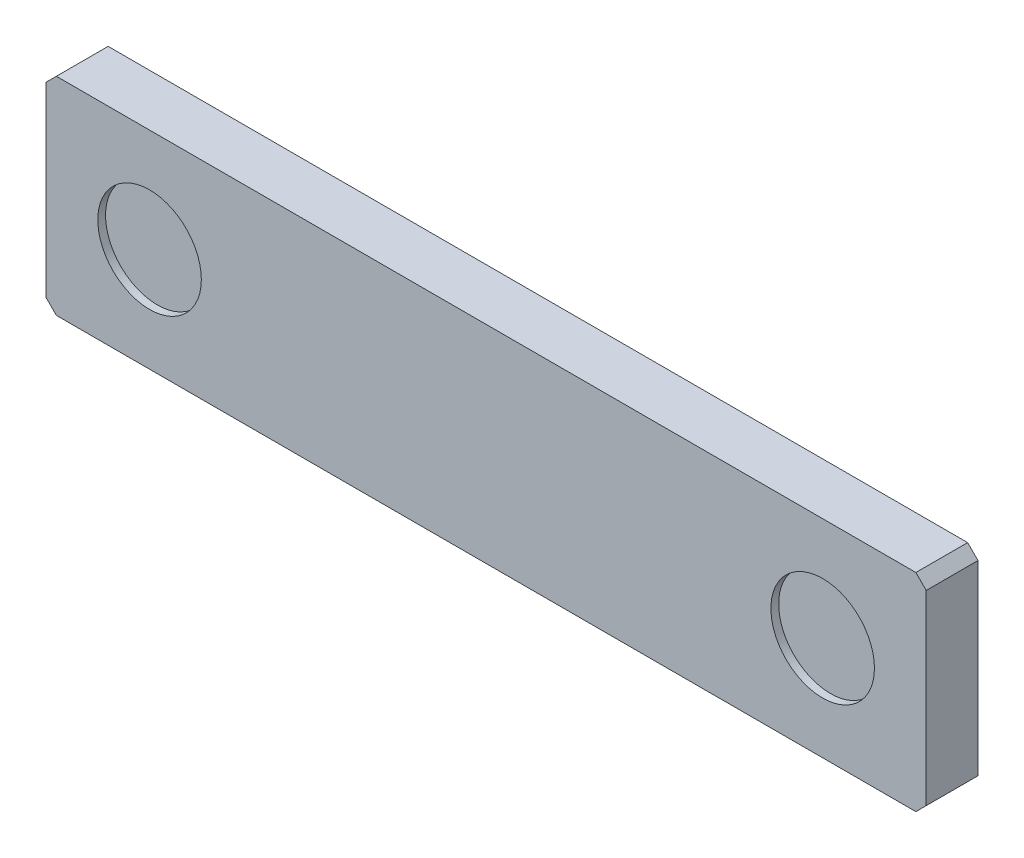
SolidWorks part; units mm, degrees
ref_plane "前视基准面" through (0, 0, 0) normal (0, 0, 1) x (1, 0, 0)
ref_plane "上视基准面" through (0, 0, 0) normal (0, 1, 0) x (1, 0, 0)
ref_plane "右视基准面" through (0, 0, 0) normal (1, 0, 0) x (0, 0, -1)
sketch "草图1" plane through (0, 0, 0) normal (0, 0, 1) x (1, 0, 0)
  line L1 (-85, -20) -> (85, -20)
  line L2 (-85, -20) -> (-85, 20)
  line L3 (-85, 20) -> (85, 20)
  line L4 (85, -20) -> (85, 20)
  line L5 (-85, -20) -> (85, 20) construction
  line L6 (-85, 20) -> (85, -20) construction
  point P0 (0, 0)
  dimension "D1" = 170
  dimension "D2" = 40
extrude "凸台-拉伸1" add sketch "草图1" along normal blind 10
sketch "草图2" plane through (0, 0, 10) normal (0, 0, 1) x (1, 0, 0)
  circle A0 centre (-65, 0) radius 10
  circle A1 centre (65, 0) radius 10
extrude "切除-拉伸1" cut sketch "草图2" against normal blind 1.5
chamfer "倒角1" distance 2 angle 45 4 edges at (-85, -20, 5) (85, -20, 5) (85, 20, 5) (-85, 20, 5)
equation "\"D2@草图2\"=\"D1@草图2\""
